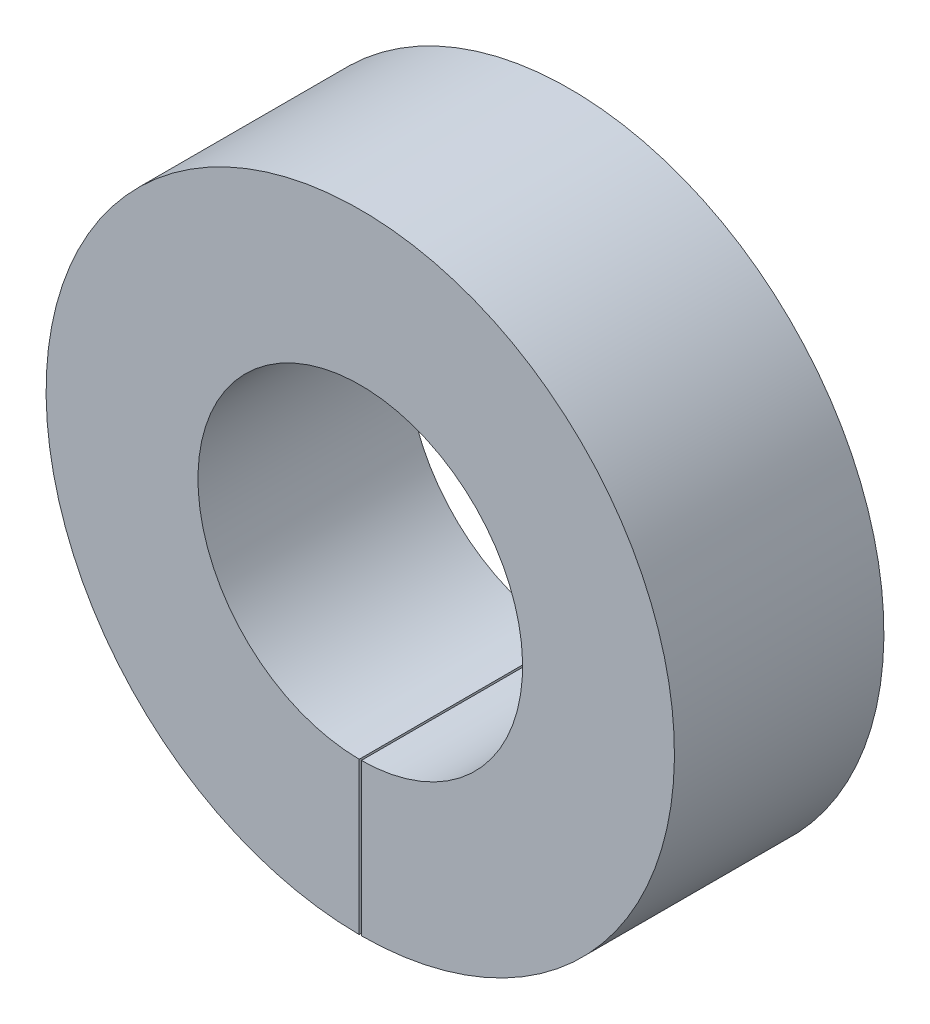
from build123d import *

# Parameters (mm, degrees)
SKETCH1_R           = 15
SKETCH1_R_2         = 7.75
BOSS_EXTRUDE1_DEPTH = 10
SKETCH2_W           = 0.1
SKETCH2_H           = 22.468635184
CUT_EXTRUDE1_DEPTH  = 24.452078799


with BuildPart() as part:
    # Sketch1 → Boss-Extrude1 (new body)
    with BuildSketch(Plane.XY):
        Circle(SKETCH1_R)
        Circle(SKETCH1_R_2, mode=Mode.SUBTRACT)
    extrude(amount=BOSS_EXTRUDE1_DEPTH)

    # Sketch2 → Cut-Extrude1 (cut, through all)
    with BuildSketch(Plane.XY.offset(10)):
        with Locations((0, -7.75)):
            Rectangle(SKETCH2_W, SKETCH2_H)
    extrude(amount=-CUT_EXTRUDE1_DEPTH, mode=Mode.SUBTRACT)


solid = part.part
